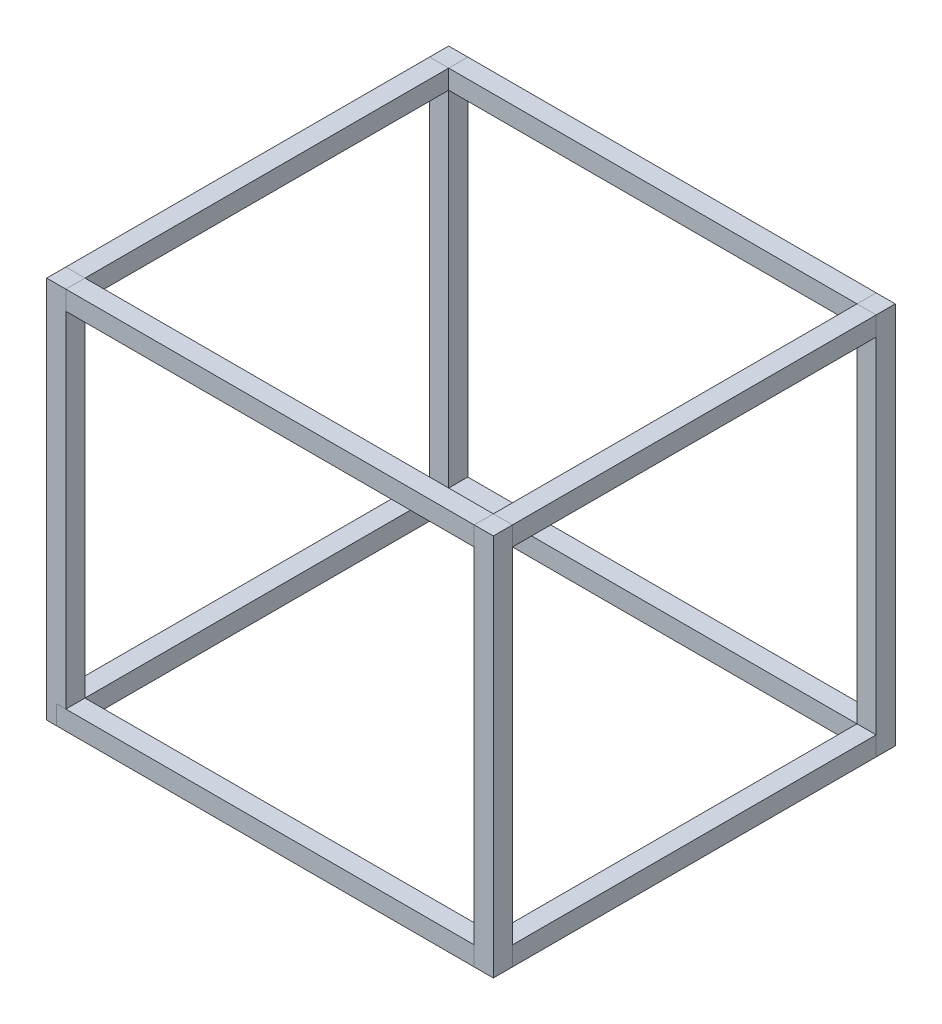
SolidWorks part; units mm, degrees
ref_plane "Front Plane" through (0, 0, 0) normal (0, 0, 1) x (1, 0, 0)
ref_plane "Top Plane" through (0, 0, 0) normal (0, 1, 0) x (1, 0, 0)
ref_plane "Right Plane" through (0, 0, 0) normal (1, 0, 0) x (0, 0, -1)
other "Configuration Table"
sketch3d "3DSketch1"
  line L0 (670, 570, 0) -> (670, 570, 600)
  line L1 (0, 0, 0) -> (670, 0, 0)
  line L2 (0, 0, 0) -> (0, 570, 0)
  line L3 (0, 570, 0) -> (670, 570, 0)
  line L4 (670, 0, 0) -> (670, 570, 0)
  line L5 (670, 0, 0) -> (670, 0, 600)
  line L6 (0, 570, 0) -> (0, 570, 600)
  line L7 (0, 0, 0) -> (0, 0, 600)
  line L9 (0, 570, 600) -> (670, 570, 600)
  line L10 (0, 570, 600) -> (0, 0, 600)
  line L11 (0, 0, 600) -> (670, 0, 600)
  line L12 (670, 570, 600) -> (670, 0, 600)
  dimension "D1" = 570
  dimension "D2" = 670
  dimension "D3" = 600
other "Square bar 30(1)"
ref_plane "Plane2" through (0, 570, 600) normal (0, -1, 0) x (1, 0, 0)
sketch "Sketch1" plane through (0, 570, 600) normal (0, -1, 0) x (1, 0, 0)
  line L1 (15, -15) -> (15, 15)
  line L2 (15, 15) -> (-15, 15)
  line L3 (-15, 15) -> (-15, -15)
  line L4 (-15, -15) -> (15, -15)
  circle A0 centre (0, 0) radius 15 construction
  point P1 (0, 15)
  point P7 (0, 0)
  point P8 (0, -15)
  point P9 (-15, 0)
  point P10 (15, 0)
  point P11 (0, 0)
  dimension "d" = 30
other "Square bar 30(2)"
ref_plane "Plane3" through (0, 0, 600) normal (1, 0, 0) x (0, 0, -1)
sketch "Sketch11" plane through (0, 0, 600) normal (1, 0, 0) x (0, 0, -1)
  line L1 (15, -15) -> (15, 15)
  line L2 (15, 15) -> (-15, 15)
  line L3 (-15, 15) -> (-15, -15)
  line L4 (-15, -15) -> (15, -15)
  circle A0 centre (0, 0) radius 15 construction
  point P1 (0, 15)
  point P7 (0, 0)
  point P8 (0, -15)
  point P9 (-15, 0)
  point P10 (15, 0)
  point P11 (0, 0)
  dimension "d" = 30
other "Trim/extend 3"
